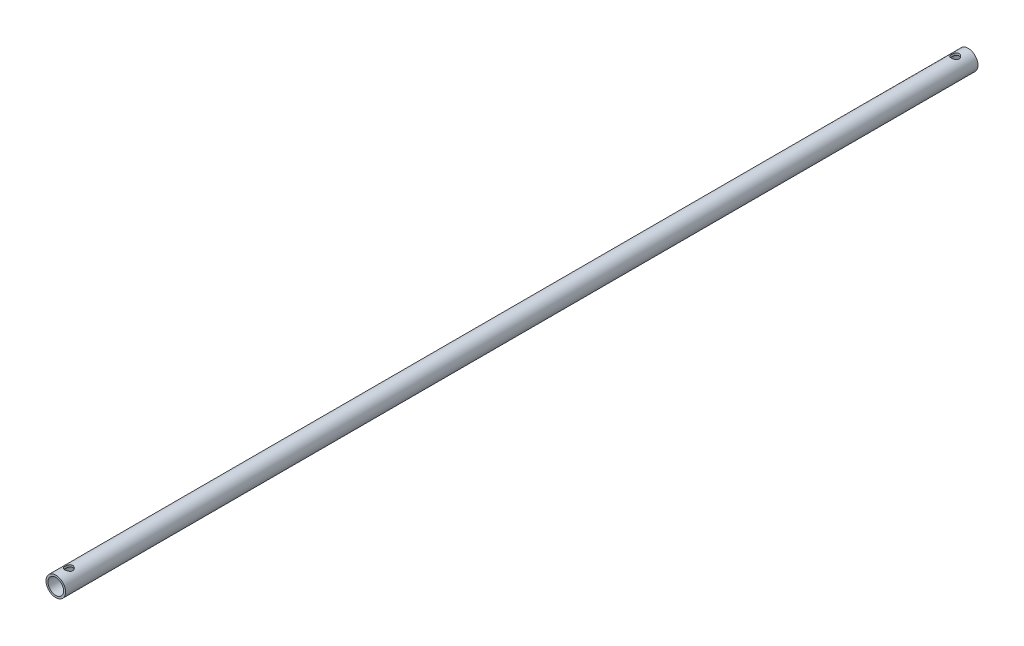
from build123d import *

# Parameters (mm, degrees)
SKETCH1_R               = 7.5
SKETCH1_R_2             = 6
BOSS_EXTRUDE1_DEPTH     = 700
CUT_EXTRUDE1_DEPTH      = 701.080352531
CUT_EXTRUDE1_DEPTH_BACK = 701.080352531
SKETCH2_R               = 3


with BuildPart() as part:
    # Sketch1 → Boss-Extrude1 (new body)
    with BuildSketch(Plane.XY):
        Circle(SKETCH1_R)
        Circle(SKETCH1_R_2, mode=Mode.SUBTRACT)
    extrude(amount=BOSS_EXTRUDE1_DEPTH)

    # Sketch2 → Cut-Extrude1 (cut, two sides: drawn at the far end of the back side and taken through both)
    with BuildSketch(Plane(origin=(0, 0, 0), x_dir=(1, 0, 0), z_dir=(0, 1, 0)).offset(-CUT_EXTRUDE1_DEPTH_BACK)):
        with Locations(Location((0, -10, 0), (0, 0, 270))):
            Circle(SKETCH2_R)
        with Locations(Location((0, -690, 0), (0, 0, 270))):
            Circle(SKETCH2_R)
    extrude(amount=CUT_EXTRUDE1_DEPTH + CUT_EXTRUDE1_DEPTH_BACK, mode=Mode.SUBTRACT)


solid = part.part
